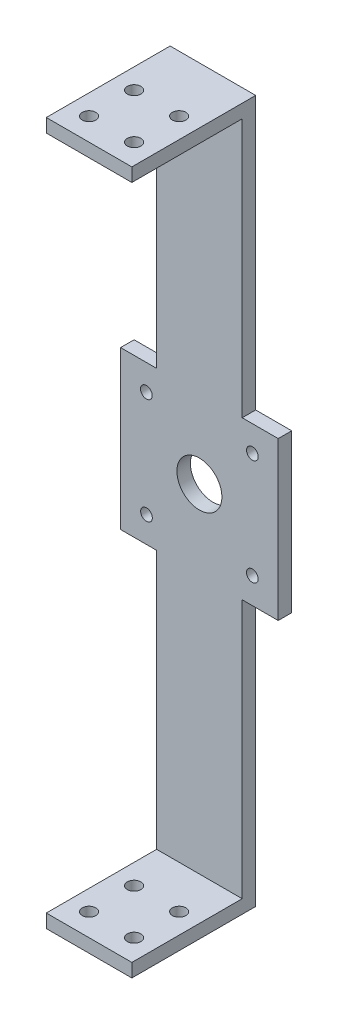
from build123d import *

# Parameters (mm, degrees)
SKETCH_1_W          = 38
SKETCH_1_H          = 55
EXTRUDE_1_DEPTH     = 6
SKETCH_2_R          = 3
CUT_EXTRUDE_1_DEPTH = 16
SKETCH_3_W          = 38
SKETCH_3_H          = 6
EXTRUDE_2_DEPTH     = 300
EXTRUDE_START       = 6
SKETCH_5_R          = 3
EXTRUDE_3_DEPTH     = 6
SKETCH_6_W          = 70
SKETCH_6_H          = 70
EXTRUDE_4_DEPTH     = 6
SKETCH_7_R          = 2.6
SKETCH_7_R_2        = 10
CUT_EXTRUDE_2_DEPTH = 10


with BuildPart() as part:
    # 草图1 → 凸台-拉伸1 (new body)
    with BuildSketch(Plane(origin=(0, 0, 0), x_dir=(1, 0, 0), z_dir=(0, 1, 0))):
        Rectangle(SKETCH_1_W, SKETCH_1_H)
    extrude(amount=EXTRUDE_1_DEPTH)

    # 草图2 → 切除-拉伸1 (cut)
    with BuildSketch(Plane(origin=(0, 6, 0), x_dir=(1, 0, 0), z_dir=(0, 1, 0))):
        with Locations(Location((-10, 2.5, 0), (0, 0, 270))):
            Circle(SKETCH_2_R)
        with Locations(Location((10, 2.5, 0), (0, 0, 270))):
            Circle(SKETCH_2_R)
        with Locations(Location((10, -17.5, 0), (0, 0, 270))):
            Circle(SKETCH_2_R)
        with Locations(Location((-10, -17.5, 0), (0, 0, 270))):
            Circle(SKETCH_2_R)
    extrude(amount=-CUT_EXTRUDE_1_DEPTH, mode=Mode.SUBTRACT)

    # 草图3 → 凸台-拉伸2 (add)
    with BuildSketch(Plane(origin=(0, 6, 0), x_dir=(1, 0, 0), z_dir=(0, 1, 0))):
        with Locations((0, 24.5)):
            Rectangle(SKETCH_3_W, SKETCH_3_H)
    extrude(amount=EXTRUDE_2_DEPTH)

    # 草图5 → 凸台-拉伸3 (add)
    with BuildSketch(Plane(origin=(0, 306, 0), x_dir=(1, 0, 0), z_dir=(0, 1, 0)).offset(EXTRUDE_START)):
        Polygon((-19, 27.5), (-19, 21.5), (-19, -27.5), (19, -27.5), (19, 21.5), (19, 27.5), align=None)
        with Locations(Location((-10, 2.5, 0), (0, 0, 270))):
            Circle(SKETCH_5_R, mode=Mode.SUBTRACT)
        with Locations(Location((10, 2.5, 0), (0, 0, 270))):
            Circle(SKETCH_5_R, mode=Mode.SUBTRACT)
        with Locations(Location((-10, -17.5, 0), (0, 0, 270))):
            Circle(SKETCH_5_R, mode=Mode.SUBTRACT)
        with Locations(Location((10, -17.5, 0), (0, 0, 270))):
            Circle(SKETCH_5_R, mode=Mode.SUBTRACT)
    extrude(amount=-EXTRUDE_3_DEPTH)

    # 草图6 → 凸台-拉伸4 (add)
    with BuildSketch(Plane(origin=(0, 0, -27.5), x_dir=(-1, 0, 0), z_dir=(0, 0, -1))):
        with Locations((0, 156)):
            Rectangle(SKETCH_6_W, SKETCH_6_H)
    extrude(amount=-EXTRUDE_4_DEPTH)

    # 草图7 → 切除-拉伸2 (cut)
    with BuildSketch(Plane(origin=(0, 0, -27.5), x_dir=(-1, 0, 0), z_dir=(0, 0, -1))):
        with Locations((23.545, 179.545)):
            Circle(SKETCH_7_R)
        with Locations((23.5, 132.5)):
            Circle(SKETCH_7_R)
        with Locations((-23.5, 132.5)):
            Circle(SKETCH_7_R)
        with Locations((-23.545, 179.545)):
            Circle(SKETCH_7_R)
        with Locations((0, 156)):
            Circle(SKETCH_7_R_2)
    extrude(amount=-CUT_EXTRUDE_2_DEPTH, mode=Mode.SUBTRACT)


solid = part.part
